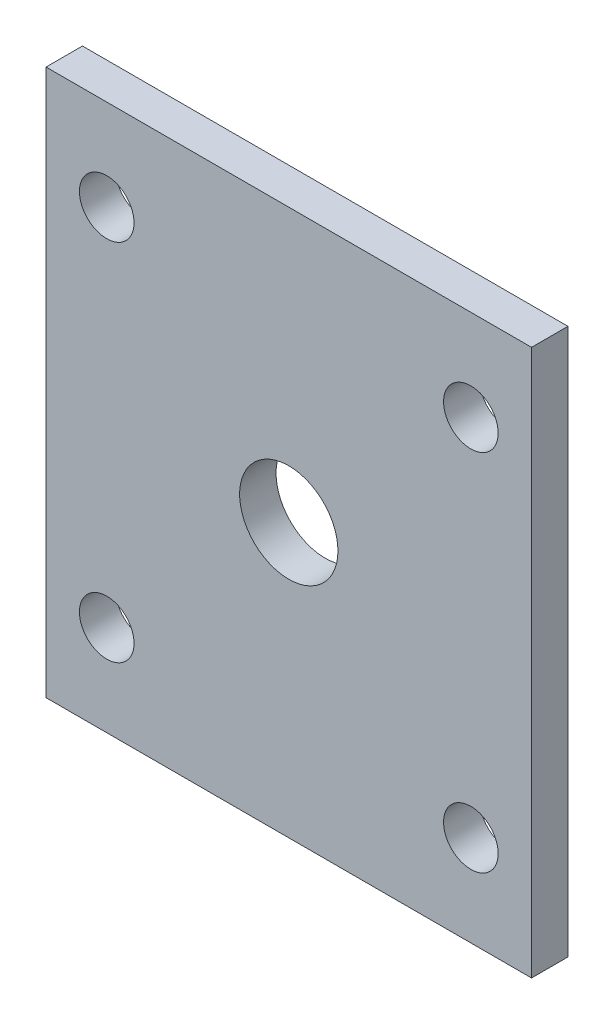
from build123d import *

# Parameters (mm, degrees)
SKETCH_1_W          = 80
SKETCH_1_H          = 90
EXTRUDE_1_DEPTH     = 3
SKETCH_2_R          = 4.5
SKETCH_2_R_2        = 8.1
CUT_EXTRUDE_1_DEPTH = 13


with BuildPart() as part:
    # 草图1 → 凸台-拉伸1 (new, symmetric)
    with BuildSketch(Plane.XY):
        Rectangle(SKETCH_1_W, SKETCH_1_H)
    extrude(amount=EXTRUDE_1_DEPTH, both=True)

    # 草图2 → 切除-拉伸1 (cut, symmetric)
    with BuildSketch(Plane.XY):
        with Locations((-30, -30)):
            Circle(SKETCH_2_R)
        with Locations((-30, 30)):
            Circle(SKETCH_2_R)
        with Locations((30, -30)):
            Circle(SKETCH_2_R)
        with Locations((30, 30)):
            Circle(SKETCH_2_R)
        Circle(SKETCH_2_R_2)
    extrude(amount=CUT_EXTRUDE_1_DEPTH, both=True, mode=Mode.SUBTRACT)


solid = part.part
